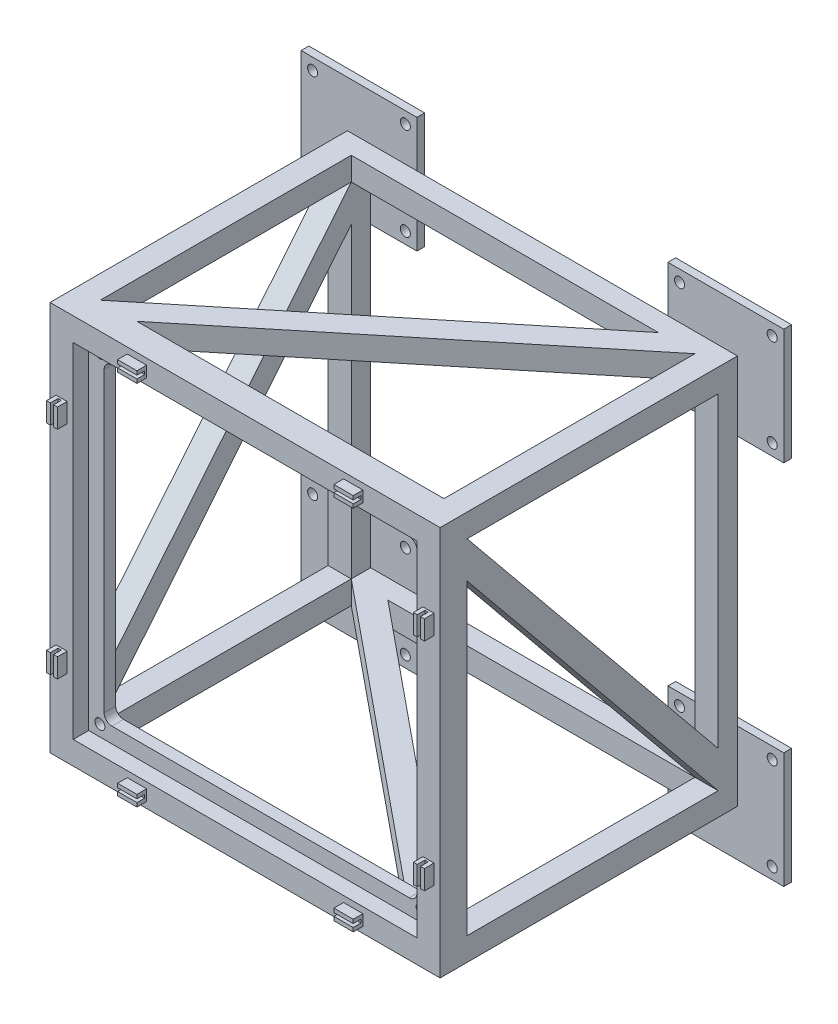
SolidWorks part; units mm, degrees
ref_plane "Front Plane" through (0, 0, 0) normal (0, 0, 1) x (1, 0, 0)
ref_plane "Top Plane" through (0, 0, 0) normal (0, 1, 0) x (1, 0, 0)
ref_plane "Right Plane" through (0, 0, 0) normal (1, 0, 0) x (0, 0, -1)
sketch "Sketch1" plane through (0, 0, 0) normal (0, 0, 1) x (1, 0, 0)
  line L1 (505, 505) -> (-505, 505)
  line L2 (505, 505) -> (505, -505)
  line L3 (505, -505) -> (-505, -505)
  line L4 (-505, 505) -> (-505, -505)
  line L5 (505, 505) -> (-505, -505) construction
  line L6 (505, -505) -> (-505, 505) construction
  point P0 (0, 0)
  dimension "D1" = 1010
  dimension "D2" = 1010
extrude "Boss-Extrude1" add sketch "Sketch1" along normal blind 770
sketch "Sketch2" plane through (0, 0, 0) normal (0, 1, 0) x (1, 0, 0)
  line L0 (505, 0) -> (-505, 0) construction
  line L1 (-445, -50) -> (445, -50)
  line L2 (-445, -50) -> (-445, -700)
  line L3 (-445, -700) -> (445, -700)
  line L4 (445, -50) -> (445, -700)
  line L5 (-445, -50) -> (445, -700) construction
  line L6 (-445, -700) -> (445, -50) construction
  line L7 (-505, -770) -> (-505, 0) construction
  line L8 (505, -770) -> (-505, -770) construction
  line L9 (505, -770) -> (505, 0) construction
  point P0 (0, -375)
  dimension "D1" = 50
  dimension "D2" = 60
  dimension "D3" = 70
  dimension "D4" = 60
extrude "Cut-Extrude1" cut sketch "Sketch2" against normal mid plane 890
sketch "Sketch3" plane through (-505, 0, 0) normal (-1, 0, 0) x (0, 0, 1)
  line L0 (700, -350.1952) -> (50, 445)
  line L1 (770, 505) -> (770, -505) construction
  line L2 (0, 505) -> (0, 411.7125)
  line L3 (0, 505) -> (0, -505) construction
  line L4 (50, 350.1952) -> (700, -445)
  line L5 (700, -350.1952) -> (700, 445)
  line L6 (700, 445) -> (50, 445)
  line L7 (50, 350.1952) -> (50, -445)
  line L8 (50, -445) -> (700, -445)
  line L9 (770, -505) -> (0, -505) construction
  line L10 (770, 505) -> (0, 505) construction
  dimension "D1" = 60
  dimension "D2" = 60
  dimension "D3" = 50
  dimension "D4" = 60
  dimension "D5" = 70
  dimension "D6" = 70
  dimension "D7" = 50
extrude "Cut-Extrude2" cut sketch "Sketch3" against normal blind 60 contours L5 L6 L0 | L7 L8 L4
sketch "Sketch4" plane through (0, 0, 0) normal (0, 1, 0) x (1, 0, 0)
  line L1 (0, 0) -> (0, -390.6952) construction
pattern_circular "CirPattern2" count 4 over 360 about axis through (0, 0, 0) along (0, 0, 1) of "Cut-Extrude2"
sketch "Sketch5" plane through (0, 0, 770) normal (0, 0, 1) x (1, 0, 0)
  line L1 (445, 445) -> (-445, 445)
  line L2 (445, 445) -> (445, -445)
  line L3 (445, -445) -> (-445, -445)
  line L4 (-445, 445) -> (-445, -445)
  line L5 (445, 445) -> (-445, -445) construction
  line L6 (445, -445) -> (-445, 445) construction
  point P0 (0, 0)
  dimension "D1" = 890
  dimension "D2" = 890
extrude "Cut-Extrude3" cut sketch "Sketch5" against normal blind 1065
sketch "Sketch6" plane through (0, 0, 700) normal (0, 0, -1) x (-1, 0, 0)
  line L0 (-445, -445) -> (445, -445) construction
  line L1 (405, 405) -> (-405, 405)
  line L2 (405, 405) -> (405, -405)
  line L3 (405, -405) -> (-405, -405)
  line L4 (-405, 405) -> (-405, -405)
  line L5 (405, 405) -> (-405, -405) construction
  line L6 (405, -405) -> (-405, 405) construction
  line L7 (445, -445) -> (445, 445) construction
  line L8 (-445, 445) -> (-445, -445) construction
  line L9 (445, 445) -> (-445, 445) construction
  line L10 (-445, -445) -> (445, -445)
  line L11 (445, -445) -> (445, 445)
  line L12 (-445, 445) -> (-445, -445)
  line L13 (445, 445) -> (-445, 445)
  point P0 (0, 0)
  dimension "D1" = 810
  dimension "D2" = 810
extrude "Boss-Extrude2" add sketch "Sketch6" against normal blind 30
fillet "Fillet1" radius 20 4 edges at (-405, -405, 715) (405, -405, 715) (405, 405, 715) (-405, 405, 715)
sketch "Sketch7" plane through (0, 0, 730) normal (0, 0, 1) x (1, 0, 0)
  circle A0 centre (-416, 416) radius 13
  circle A1 centre (416, 416) radius 13
  circle A2 centre (416, -416) radius 13
  circle A3 centre (-416, -416) radius 13
  dimension "D5" = 26
  dimension "D1" = 832
  dimension "D2" = 416
  dimension "D3" = 832
  dimension "D4" = 416
extrude "Cut-Extrude4" cut sketch "Sketch7" against normal blind 30
sketch "Sketch8" plane through (0, 0, 0) normal (0, 0, -1) x (-1, 0, 0)
  line L0 (-505, -505) -> (-505, 505) construction
  line L1 (-325, -325) -> (-625, -325)
  line L2 (-325, -325) -> (-325, -625)
  line L3 (-325, -625) -> (-625, -625)
  line L4 (-625, -325) -> (-625, -625)
  line L5 (-325, -325) -> (-625, -625) construction
  line L6 (-325, -625) -> (-625, -325) construction
  line L7 (505, -505) -> (-505, -505) construction
  circle A0 centre (-595, -355) radius 13
  circle A1 centre (-355, -355) radius 13
  circle A2 centre (-595, -595) radius 13
  circle A3 centre (-355, -595) radius 13
  point P0 (-475, -475)
  dimension "D9" = 26
  dimension "D1" = 300
  dimension "D2" = 300
  dimension "D3" = 120
  dimension "D4" = 120
  dimension "D5" = 240
  dimension "D6" = 240
  dimension "D7" = 120
  dimension "D8" = 120
extrude "Boss-Extrude3" add sketch "Sketch8" along normal blind 20
pattern_circular "CirPattern3" count 4 over 360 about axis through (0, 0, 0) along (0, 0, 1) of "Boss-Extrude3"
sketch "Sketch9" plane through (0, 0, 770) normal (0, 0, 1) x (1, 0, 0)
  line L0 (-445, -445) -> (445, -445) construction
  line L1 (-305, -460.75) -> (-255, -460.75)
  line L2 (-305, -460.75) -> (-305, -489.25)
  line L3 (-305, -489.25) -> (-255, -489.25)
  line L4 (-255, -460.75) -> (-255, -489.25)
  line L5 (-305, -460.75) -> (-255, -489.25) construction
  line L6 (-305, -489.25) -> (-255, -460.75) construction
  line L8 (-505, 505) -> (-505, -505) construction
  line L9 (0, 0) -> (0, -109.2116) construction
  line L10 (305, -489.25) -> (255, -460.75) construction
  line L11 (305, -460.75) -> (255, -489.25) construction
  line L12 (255, -460.75) -> (255, -489.25)
  line L13 (305, -489.25) -> (255, -489.25)
  line L14 (305, -460.75) -> (305, -489.25)
  line L15 (305, -460.75) -> (255, -460.75)
  line L16 (-460.75, 305) -> (-489.25, 305)
  line L17 (-460.75, 305) -> (-460.75, 255)
  line L18 (-460.75, 255) -> (-489.25, 255)
  line L19 (-489.25, 305) -> (-489.25, 255)
  line L20 (-460.75, -255) -> (-489.25, -255)
  line L21 (-489.25, -305) -> (-489.25, -255)
  line L22 (-460.75, -305) -> (-489.25, -305)
  line L23 (-460.75, -305) -> (-460.75, -255)
  line L24 (305, 460.75) -> (305, 489.25)
  line L25 (305, 460.75) -> (255, 460.75)
  line L26 (255, 460.75) -> (255, 489.25)
  line L27 (305, 489.25) -> (255, 489.25)
  line L28 (-255, 460.75) -> (-255, 489.25)
  line L29 (-305, 489.25) -> (-255, 489.25)
  line L30 (-305, 460.75) -> (-305, 489.25)
  line L31 (-305, 460.75) -> (-255, 460.75)
  line L32 (460.75, -305) -> (489.25, -305)
  line L33 (460.75, -305) -> (460.75, -255)
  line L34 (460.75, -255) -> (489.25, -255)
  line L35 (489.25, -305) -> (489.25, -255)
  line L36 (460.75, 255) -> (489.25, 255)
  line L37 (489.25, 305) -> (489.25, 255)
  line L38 (460.75, 305) -> (489.25, 305)
  line L39 (460.75, 305) -> (460.75, 255)
  point P0 (-280, -475)
  point P16 (280, -475)
  point P44 (0, 0)
  dimension "D1" = 50
  dimension "D2" = 28.5
  dimension "D3" = 30
  dimension "D4" = 200
  dimension "D5" = 4
extrude "Boss-Extrude4" add sketch "Sketch9" along normal blind 25
sketch "Sketch10" plane through (0, 0, 795) normal (0, 0, 1) x (1, 0, 0)
  line L0 (-255, -489.25) -> (-255, -460.75) construction
  line L1 (340.704, -470.75) -> (-850.704, -470.75)
  line L2 (340.704, -470.75) -> (340.704, -479.25)
  line L3 (340.704, -479.25) -> (-850.704, -479.25)
  line L4 (-850.704, -470.75) -> (-850.704, -479.25)
  line L5 (340.704, -470.75) -> (-850.704, -479.25) construction
  line L6 (340.704, -479.25) -> (-850.704, -470.75) construction
  point P0 (-255, -475)
  dimension "D1" = 8.5
extrude "Cut-Extrude5" cut sketch "Sketch10" against normal blind 20
pattern_circular "CirPattern4" count 4 over 360 about axis through (0, 0, 0) along (0, 0, 1) of "Cut-Extrude5"
